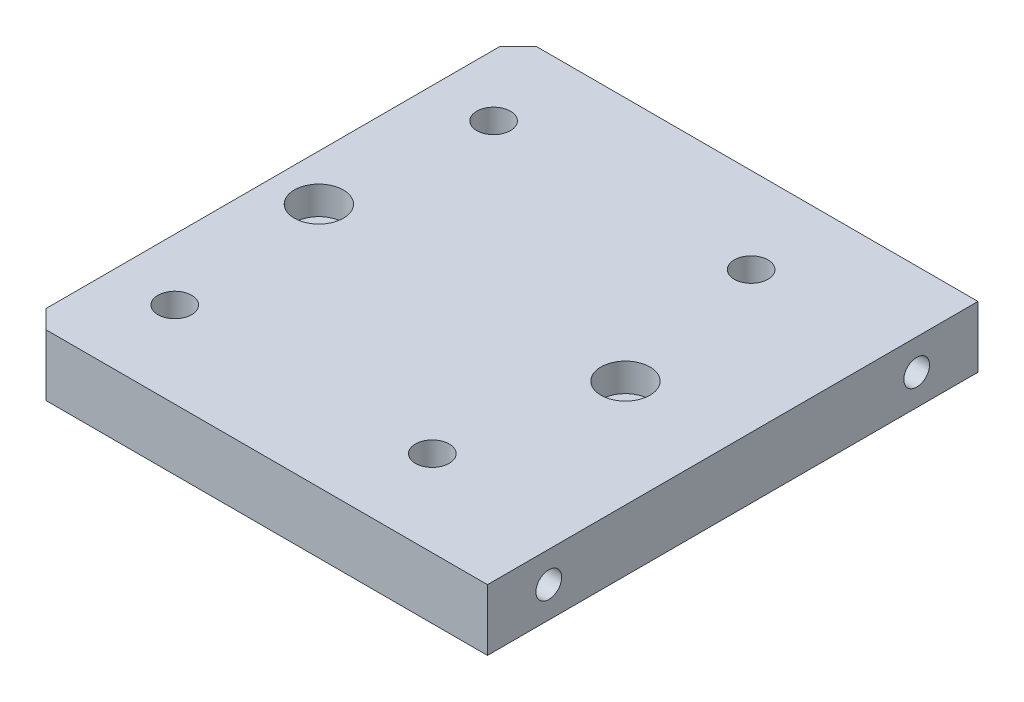
SolidWorks part; units mm, degrees
material "A6061"
ref_plane "前基準面" through (0, 0, 0) normal (0, 0, 1) x (1, 0, 0)
ref_plane "上基準面" through (0, 0, 0) normal (0, 1, 0) x (1, 0, 0)
ref_plane "右基準面" through (0, 0, 0) normal (1, 0, 0) x (0, 0, -1)
sketch "草图1" plane through (0, 0, 0) normal (0, 1, 0) x (1, 0, 0)
  line L1 (-37.5, -40) -> (37.5, -40)
  line L2 (-37.5, -40) -> (-37.5, 40)
  line L3 (-37.5, 40) -> (37.5, 40)
  line L4 (37.5, -40) -> (37.5, 40)
  line L5 (-37.5, -40) -> (37.5, 40) construction
  line L6 (-37.5, 40) -> (37.5, -40) construction
  point P0 (0, 0)
  dimension "D1" = 75
  dimension "D2" = 80
extrude "凸台-拉伸1" add sketch "草图1" along normal mid plane 10
chamfer "倒角1" distance 3 angle 45 2 edges at (-37.5, 0, 40) (-37.5, 0, -40)
hole_wizard "M5 螺纹孔1" positions "草图2" profile "草图3" tap size "M5" standard "GB"
sketch "草图2" plane through (37.5, 0, 0) normal (1, 0, 0) x (0, 0, -1)
  line L0 (0, 22.3943) -> (0, 0) construction
  point P0 (-30, 0)
  point P7 (30, 0)
  dimension "D1" = 60
sketch "草图3" plane through (37.5, 0, 30) normal (0, 1, 0) x (0, 0, -1)
  line L0 (0, 0) -> (0, 13.6618)
  line L1 (0, 13.6618) -> (2.1, 12.4)
  line L2 (2.1, 12.4) -> (2.1, 0)
  line L5 (2.1, 0) -> (0, 0)
  line L10 (0, 13.6618) -> (-2.1, 12.4) construction
  line L11 (0, -6.35) -> (0, 107.95) construction
  dimension "螺纹孔钻头直径" = 4.2
  dimension "螺纹孔钻头深度" = 12.4
  dimension "导头角度" = 118
cosmetic thread "孔螺蚊线1" parameters "D1"=10, "D2"=5
cosmetic thread "孔螺蚊线2" parameters "D1"=10, "D2"=5
hole_wizard "打孔尺寸(%根据)内六角圆柱头螺钉的类型1" positions "草图4" profile "草图5" counterbore size "M5" standard "GB" end condition through all
sketch "草图4" plane through (0, -5, 0) normal (0, 1, 0) x (1, 0, 0)
  line L0 (0, 0) -> (-56.4835, 0) construction
  line L2 (-37.5, 37) -> (-37.5, -37) construction
  point P0 (-27.5, 26)
  point P2 (14.5, 26)
  point P11 (14.5, -26)
  point P12 (-27.5, -26)
  dimension "D1" = 52
  dimension "D2" = 42
  dimension "D3" = 10
sketch "草图5" plane through (-27.5, -5, -26) normal (1, 0, 0) x (0, 0, -1)
  line L0 (0, 0) -> (0, 10)
  line L1 (0, 10) -> (2.75, 10)
  line L3 (2.75, 10) -> (2.75, 5.7)
  line L4 (2.75, 5.7) -> (5, 5.7)
  line L5 (5, 5.7) -> (5, 0)
  line L7 (5, 0) -> (0, 0)
  line L11 (0, -6.35) -> (0, 107.95) construction
  dimension "通孔孔直径" = 5.5
  dimension "通孔孔深度" = 10
  dimension "柱形沉头孔直径" = 10
  dimension "柱形沉头孔深度" = 5.7
hole_wizard "打孔尺寸(%根据)内六角圆柱头螺钉的类型2" positions "草图6" profile "草图7" counterbore size "M4" standard "GB" end condition through all
sketch "草图6" plane through (0, 5, 0) normal (0, 1, 0) x (1, 0, 0)
  line L0 (37.5, -40) -> (37.5, 40) construction
  point P0 (-30, 0)
  point P2 (20, 0)
  dimension "D1" = 50
  dimension "D2" = 17.5
sketch "草图7" plane through (-30, 5, 0) normal (1, 0, 0) x (0, 0, 1)
  line L0 (0, 0) -> (0, 10)
  line L1 (0, 10) -> (2.25, 10)
  line L3 (2.25, 10) -> (2.25, 4.6)
  line L4 (2.25, 4.6) -> (4, 4.6)
  line L5 (4, 4.6) -> (4, 0)
  line L7 (4, 0) -> (0, 0)
  line L11 (0, -6.35) -> (0, 107.95) construction
  dimension "通孔孔直径" = 4.5
  dimension "通孔孔深度" = 10
  dimension "柱形沉头孔直径" = 8
  dimension "柱形沉头孔深度" = 4.6
